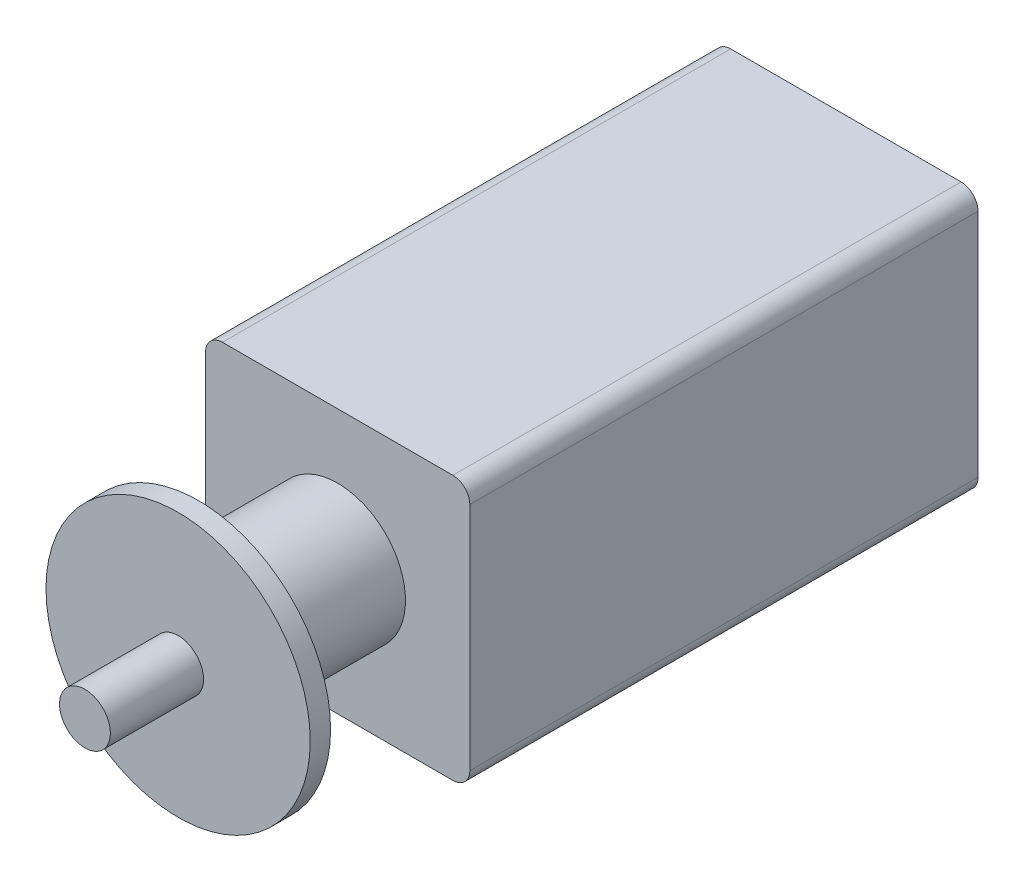
from build123d import *

# Parameters (mm, degrees)
SKETCH1_W           = 156
SKETCH1_H           = 156
BOSS_EXTRUDE1_DEPTH = 300
SKETCH2_R           = 40
BOSS_EXTRUDE2_DEPTH = 88
SKETCH3_R           = 78
BOSS_EXTRUDE3_DEPTH = 12
FILLET1_R           = 10
SKETCH4_R           = 15
BOSS_EXTRUDE4_DEPTH = 55


with BuildPart() as part:
    # Sketch1 → Boss-Extrude1 (new body)
    with BuildSketch(Plane.XY):
        with Locations((78, 78)):
            Rectangle(SKETCH1_W, SKETCH1_H)
    extrude(amount=BOSS_EXTRUDE1_DEPTH)

    # Sketch2 → Boss-Extrude2 (add)
    with BuildSketch(Plane.XY.offset(300)):
        with Locations(Location((78, 78, 0), (0, 0, 180))):
            Circle(SKETCH2_R)
    extrude(amount=BOSS_EXTRUDE2_DEPTH)

    # Sketch3 → Boss-Extrude3 (add)
    with BuildSketch(Plane.XY.offset(388)):
        with Locations((83.788071994, 78)):
            Circle(SKETCH3_R)
    extrude(amount=BOSS_EXTRUDE3_DEPTH)

    # Fillet1
    fillet1_edges = [part.edges().sort_by_distance(p)[0] for p in [
        (0, 156, 150),
        (156, 156, 150),
        (156, 0, 150),
        (0, 0, 150),
    ]]
    fillet(fillet1_edges, radius=FILLET1_R)

    # Sketch4 → Boss-Extrude4 (add)
    with BuildSketch(Plane.XY.offset(400)):
        with Locations((83.788071994, 78)):
            Circle(SKETCH4_R)
    extrude(amount=BOSS_EXTRUDE4_DEPTH)


solid = part.part
